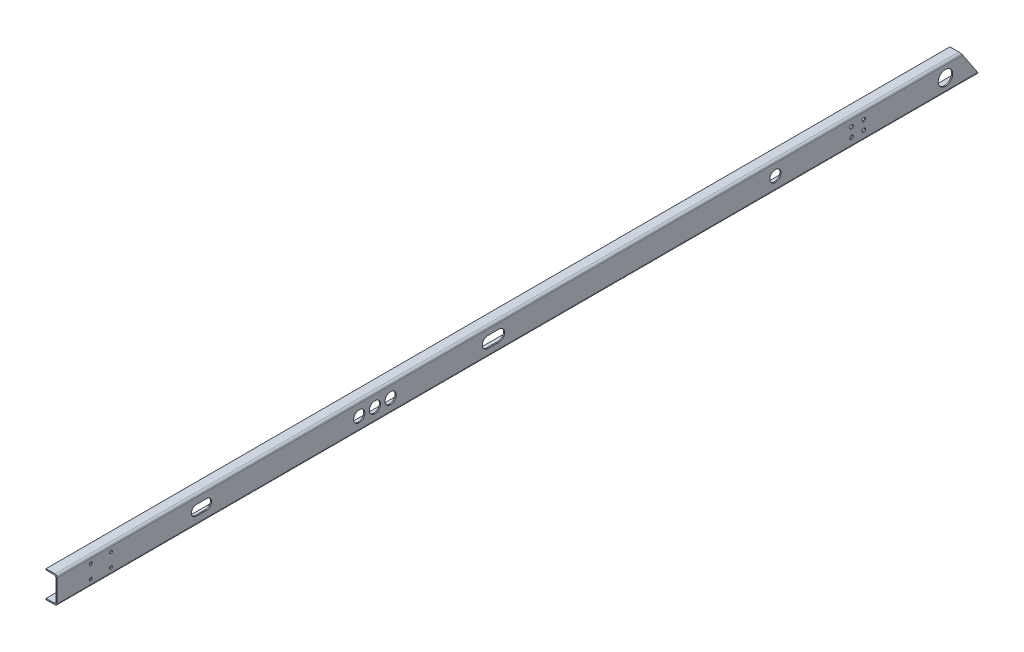
SolidWorks part; units mm, degrees
ref_plane "前视基准面" through (0, 0, 0) normal (0, 0, 1) x (1, 0, 0)
ref_plane "上视基准面" through (0, 0, 0) normal (0, 1, 0) x (1, 0, 0)
ref_plane "右视基准面" through (0, 0, 0) normal (1, 0, 0) x (0, 0, -1)
sketch "草图1" plane through (0, 0, 0) normal (0, 0, 1) x (1, 0, 0)
  line L24 (626.1756, -48.4289) -> (666.1756, -48.4289)
  line L25 (676.1756, -38.4289) -> (676.1756, 61.5711)
  line L26 (666.1756, 71.5711) -> (626.1756, 71.5711)
  line L27 (626.1756, 71.5711) -> (626.1756, 66.5711)
  line L28 (626.1756, 66.5711) -> (661.1756, 66.5711)
  line L29 (671.1756, 56.5711) -> (671.1756, -33.4289)
  line L30 (661.1756, -43.4289) -> (626.1756, -43.4289)
  line L31 (626.1756, -43.4289) -> (626.1756, -48.4289)
  arc A12 (666.1756, -48.4289) -> (676.1756, -38.4289) centre (666.1756, -38.4289) ccw
  arc A13 (676.1756, 61.5711) -> (666.1756, 71.5711) centre (666.1756, 61.5711) ccw
  arc A14 (671.1756, 56.5711) -> (661.1756, 66.5711) centre (661.1756, 56.5711) ccw
  arc A15 (661.1756, -43.4289) -> (671.1756, -33.4289) centre (661.1756, -33.4289) ccw
extrude "凸台-拉伸1" add sketch "草图1" along normal blind 4120
sketch "草图2" plane through (676.1756, 0, 0) normal (1, 0, 0) x (0, 0, -1)
  line L14 (-3497.5, 34.0711) -> (-3452.5, 34.0711)
  line L15 (-3497.5, -10.9289) -> (-3452.5, -10.9289)
  line L23 (-2195, 36.5711) -> (-2145, 36.5711)
  line L24 (-2145, -13.4289) -> (-2195, -13.4289)
  circle A0 centre (-3985, -18.4289) radius 6.5
  circle A1 centre (-3985, 41.5711) radius 6.5
  circle A2 centre (-3895, 41.5711) radius 6.5
  circle A3 centre (-3895, -18.4289) radius 6.5
  arc A4 (-3452.5, -10.9289) -> (-3452.5, 34.0711) centre (-3452.5, 11.5711) ccw
  arc A5 (-3497.5, 34.0711) -> (-3497.5, -10.9289) centre (-3497.5, 11.5711) ccw
  circle A6 centre (-2770, 11.5711) radius 25
  circle A7 centre (-2700, 11.5711) radius 25
  circle A8 centre (-2630, 11.5711) radius 25
  circle A9 centre (-150, 11.5711) radius 22.5
  arc A10 (-2195, 36.5711) -> (-2195, -13.4289) centre (-2195, 11.5711) ccw
  arc A11 (-2145, 36.5711) -> (-2145, -13.4289) centre (-2145, 11.5711) cw
  circle A12 centre (-570, 31.5711) radius 8
  circle A13 centre (-515, 31.5711) radius 8
  circle A14 centre (-570, -8.4289) radius 8
  circle A15 centre (-515, -8.4289) radius 8
extrude "切除-拉伸2" cut sketch "草图2" against normal blind 10
sketch "草图3" plane through (676.1756, 0, 0) normal (1, 0, 0) x (0, 0, -1)
  line L1 (-4120, 61.5711) -> (0, 61.5711) construction
  line L4 (-910, 61.5711) -> (-910, -38.4289)
  line L5 (-4120, -38.4289) -> (0, -38.4289) construction
  circle A0 centre (-910, 11.5711) radius 25
extrude "切除-拉伸3" cut sketch "草图3" against normal blind 10 contours L4 A0 | L4 A0
sketch "草图4" plane through (676.1756, 0, 0) normal (1, 0, 0) x (0, 0, -1)
  circle A7 centre (-3880, 41.5711) radius 6.5
  circle A9 centre (-3970, 41.5711) radius 6.5
  circle A10 centre (-3970, -18.4289) radius 6.5
  circle A11 centre (-3880, -18.4289) radius 6.5
extrude "切除-拉伸4" cut sketch "草图4" against normal blind 10
sketch "草图5" plane through (676.1756, 0, 0) normal (1, 0, 0) x (0, 0, -1)
  line L0 (-3911.284, 53.9053) -> (-3903.726, -30.7435)
  line L1 (-3977.5291, 52.1396) -> (-3977.5291, -29.395)
  line L2 (-3887.4117, -18.4289) -> (-3887.4117, -30.7435)
  line L3 (-3887.4117, -30.7435) -> (-3887.4117, 56.0367)
  line L4 (-3887.4117, 56.0367) -> (-3911.284, 53.9053)
  line L5 (-3903.726, -30.7435) -> (-3887.4117, -30.7435)
  line L6 (-3977.5291, -29.395) -> (-4000.2755, -29.395)
  line L7 (-4000.2755, -29.395) -> (-4000.2755, 52.1396)
  line L8 (-4000.2755, 52.1396) -> (-3977.5291, 52.1396)
  circle M22 centre (-3895, -18.4289) radius 6.5
  circle M23 centre (-3895, 41.5711) radius 6.5
  circle M24 centre (-3985, 41.5711) radius 6.5
  circle M25 centre (-3985, -18.4289) radius 6.5
extrude "凸台-拉伸2" add sketch "草图5" against normal blind 5 contours L8 L7 L6 L1 M24 M25 | L0 L5 L2 L3 L4 M23 M22 | M24 | M25 | M22 | M23
sketch "草图6" plane through (676.1756, 0, 0) normal (1, 0, 0) x (0, 0, -1)
  circle A1 centre (-150, 11.5711) radius 32.5
extrude "切除-拉伸5" cut sketch "草图6" against normal blind 10
sketch "草图7" plane through (676.1756, 0, 0) normal (1, 0, 0) x (0, 0, -1)
  line L0 (0, 71.5711) -> (-80, 71.5711)
  line L1 (-4120, 71.5711) -> (0, 71.5711) construction
  line L2 (-80, 71.5711) -> (0, -48.4289)
  line L3 (0, -48.4289) -> (0, 71.5711)
extrude "切除-拉伸6" cut sketch "草图7" against normal blind 63
